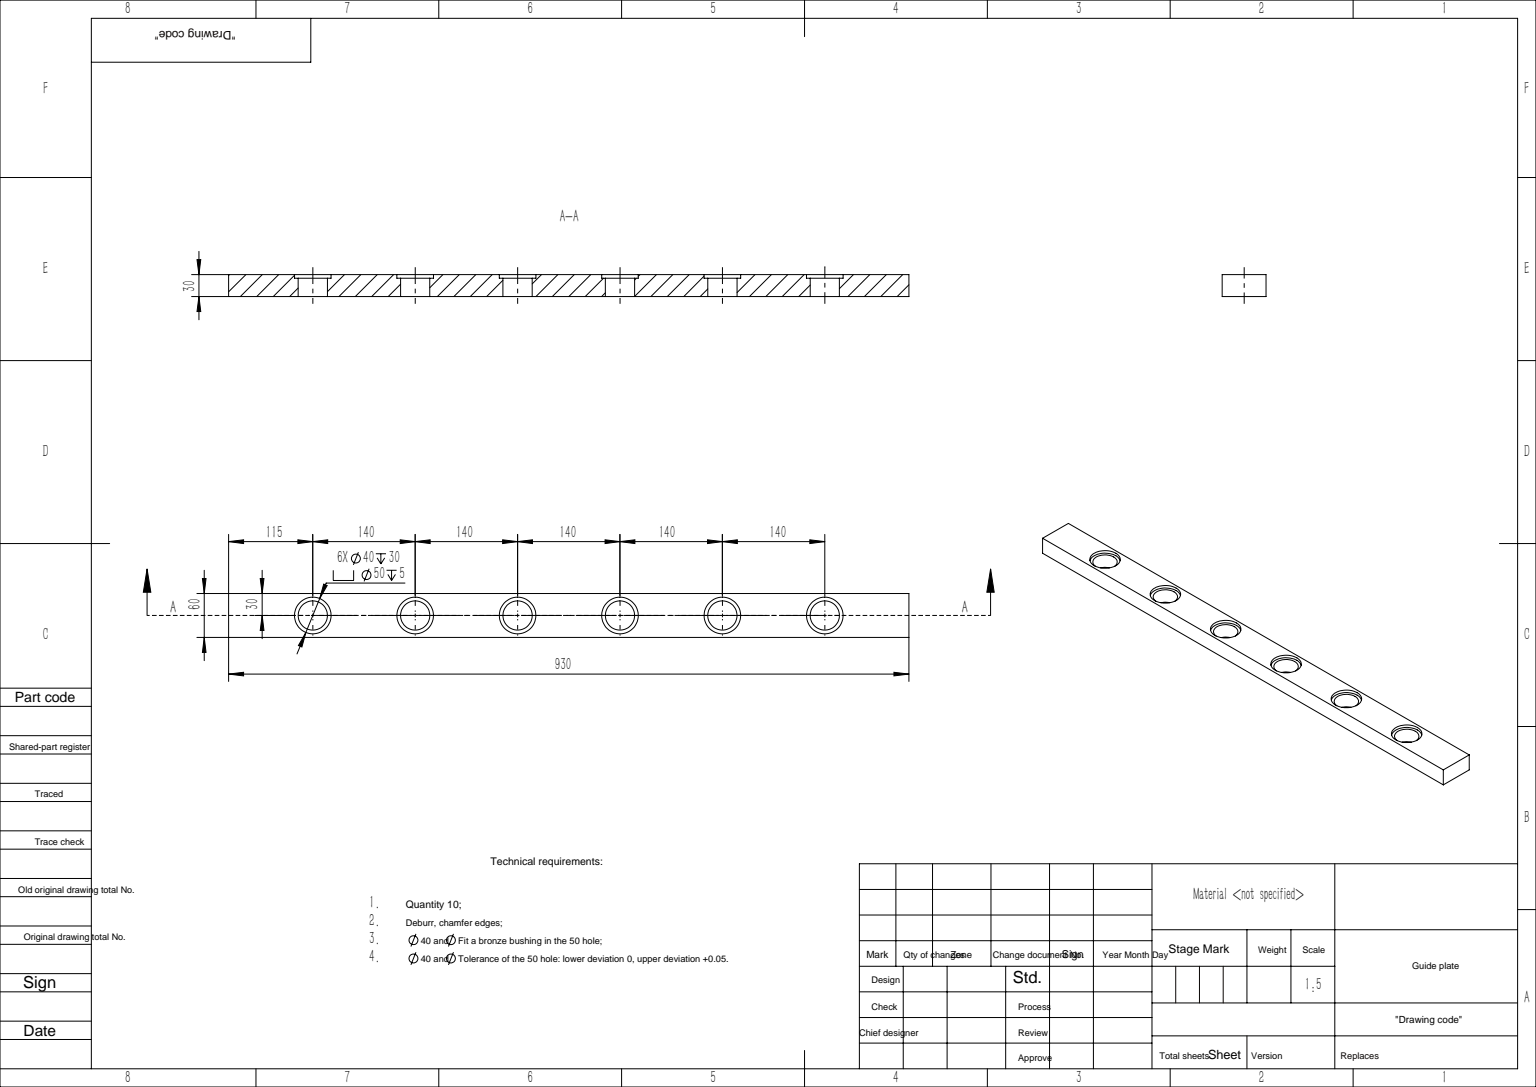
SolidWorks part; units mm, degrees
ref_plane "前视基准面" through (0, 0, 0) normal (0, 0, 1) x (1, 0, 0)
ref_plane "上视基准面" through (0, 0, 0) normal (0, 1, 0) x (1, 0, 0)
ref_plane "右视基准面" through (0, 0, 0) normal (1, 0, 0) x (0, 0, -1)
sketch "草图1" plane through (0, 0, 0) normal (0, 1, 0) x (1, 0, 0)
  line L1 (-465, -30) -> (465, -30)
  line L2 (-465, -30) -> (-465, 30)
  line L3 (-465, 30) -> (465, 30)
  line L4 (465, -30) -> (465, 30)
  line L5 (-465, -30) -> (465, 30) construction
  line L6 (-465, 30) -> (465, -30) construction
  point P0 (0, 0)
  dimension "D1" = 930
  dimension "D2" = 60
extrude "凸台-拉伸1" add sketch "草图1" along normal blind 30
sketch "草图3" plane through (0, 0, 0) normal (0, 0, 1) x (1, 0, 0)
  line L0 (350, 30) -> (375, 30)
  line L1 (-465, 30) -> (465, 30) construction
  line L2 (375, 30) -> (375, 25)
  line L3 (375, 25) -> (370, 25)
  line L4 (370, 25) -> (370, 0)
  line L5 (-465, 0) -> (465, 0) construction
  line L6 (370, 0) -> (350, 0)
  line L7 (350, 0) -> (350, 30)
  line L8 (465, 30) -> (465, 0) construction
  dimension "D1" = 25
  dimension "D2" = 5
  dimension "D3" = 20
  dimension "D4" = 115
revolve "切除-旋转1" cut sketch "草图3" angle 360 about L7
pattern_linear "阵列(线性)1" count 6 spacing 140 along (-1, 0, 0) of "切除-旋转1"
